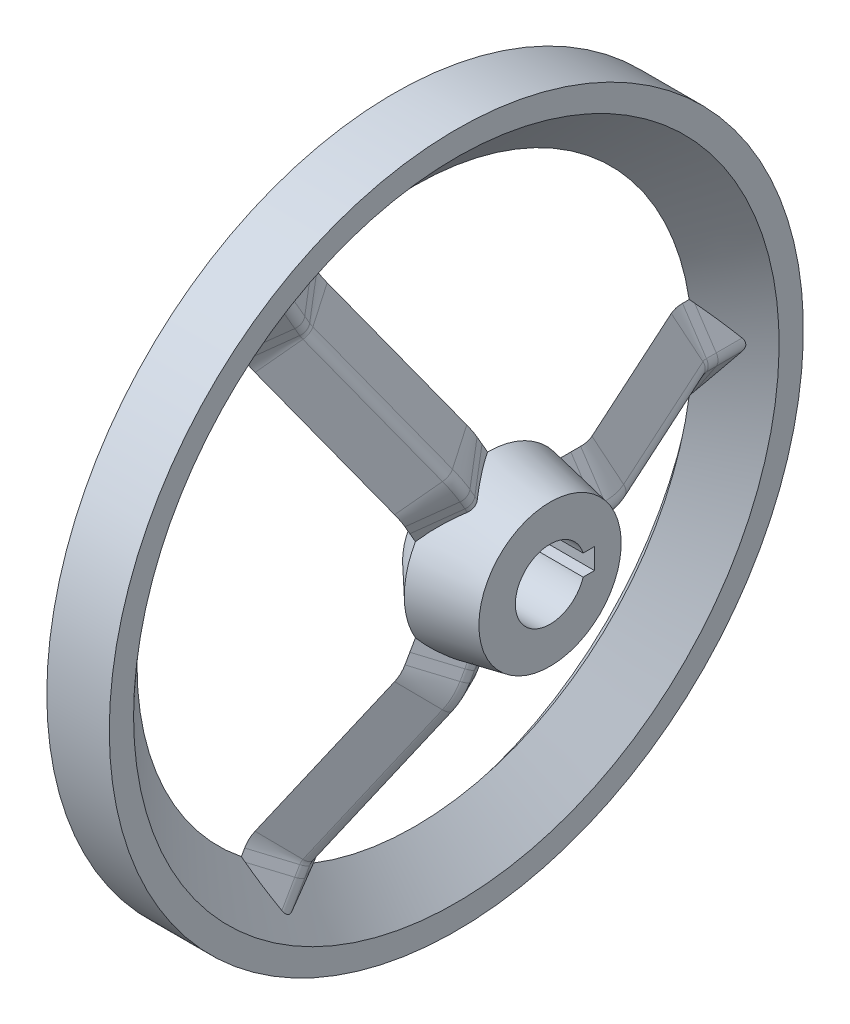
SolidWorks part; units mm, degrees
ref_plane "前视基准面" through (0, 0, 0) normal (0, 0, 1) x (1, 0, 0)
ref_plane "上视基准面" through (0, 0, 0) normal (0, 1, 0) x (1, 0, 0)
ref_plane "右视基准面" through (0, 0, 0) normal (1, 0, 0) x (0, 0, -1)
other "Configuration Table"
sketch "草图1" plane through (0, 0, 0) normal (0, 0, 1) x (1, 0, 0)
  line L0 (0, 0) -> (121.4845, 0) construction
  line L1 (0, 100) -> (0, 87.5)
  line L2 (0, 87.5) -> (6, 80)
  line L3 (6, 80) -> (18, 93)
  line L4 (18, 93) -> (18, 100)
  line L5 (18, 100) -> (0, 100)
  line L7 (27, 24) -> (45, 20.5)
  line L8 (45, 20.5) -> (45, 10)
  line L9 (45, 10) -> (18, 10)
  line L10 (18, 10) -> (18, 15.5)
  line L11 (18, 15.5) -> (27, 24)
  point P10 (18, 96.5)
  dimension "D1" = 12.5
  dimension "D2" = 18
  dimension "D3" = 6
  dimension "D4" = 7
  dimension "D5" = 200
  dimension "D6" = 27
  dimension "D7" = 48
  dimension "D8" = 160
  dimension "D9" = 20
  dimension "D10" = 10.5
  dimension "D11" = 9
  dimension "D12" = 5.5
  dimension "D13" = 45
revolve "旋转1" add sketch "草图1" angle 360 about L0
ref_plane "基准面1" through (0, 0, -14) normal (0, 0, 1) x (1, 0, 0)
sketch "草图2" plane through (0, 0, -14) normal (0, 0, 1) x (1, 0, 0)
  line L0 (0, 0) -> (44.3337, 0) construction
  line L6 (27, 12) -> (22.4808, 1.1538)
  line L7 (22.4808, -1.1538) -> (27, -12)
  line L8 (27, -24) -> (27, 24) construction
  line L9 (27, -12) -> (33.8906, -1.6641)
  line L10 (33.8906, 1.6641) -> (27, 12)
  arc A0 (33.8906, -1.6641) -> (33.8906, 1.6641) centre (31.3944, 0) ccw
  arc A1 (22.4808, 1.1538) -> (22.4808, -1.1538) centre (25.25, 0) ccw
  point P17 (35, 0)
  point P20 (22, 0)
  dimension "D1" = 13
  dimension "D2" = 24
  dimension "D5" = 3
  dimension "D3" = 5
  dimension "D4" = 12
sketch "草图3" plane through (0, 0, 0) normal (0, 1, 0) x (1, 0, 0)
  line L0 (26.0969, 30.9783) -> (6.9031, 73.0217)
  line L1 (6, 77.1747) -> (6, 80)
  line L2 (27, -24) -> (27, 24) construction
  line L3 (6, -100) -> (6, 100) construction
  line L4 (0, -100) -> (18, -100) construction
  line L5 (18, 100) -> (0, 100) construction
  line L6 (27, 24) -> (27, 14)
  line L7 (27, 26.8253) -> (27, 24)
  line L8 (6, 80) -> (6, 90)
  line L9 (45, -20.5) -> (45, 20.5) construction
  line L11 (0, 100) -> (0, -100) construction
  arc A0 (26.0969, 30.9783) -> (27, 26.8253) centre (17, 26.8253) cw
  arc A1 (6, 77.1747) -> (6.9031, 73.0217) centre (16, 77.1747) ccw
  point P22 (27, 29)
  point P25 (6, 75)
  dimension "D8" = 10
  dimension "D1" = 10
  dimension "D2" = 15
  dimension "D3" = 5
  dimension "D4" = 15
  dimension "D5" = 6
  dimension "D6" = 10
  dimension "D7" = 14
  dimension "D9" = 18
sweep "扫描4" add profiles "草图2" path "草图3"
pattern_circular "阵列(圆周)1" count 3 over 360 about axis through (0, 0, 0) along (1, 0, 0) of "扫描4"
ref_plane "基准面2" through (6, 0, 0) normal (-1, 0, 0) x (0, 0, 1)
sketch "草图4" plane through (6, 0, 0) normal (-1, 0, 0) x (0, 0, 1)
  line L1 (0, 0) -> (42.0474, 72.8283) construction
  line L2 (0, 0) -> (0, 48.3174) construction
  circle A0 centre (42.0474, 72.8283) radius 13
  dimension "D1" = 26
  dimension "D3" = 30
  dimension "D2" = 84.0949
extrude "凸台-拉伸1" add sketch "草图4" along normal up to surface (6 mm away) up to face at (0, 0, 87.5)
sketch "草图5" plane through (6, 0, 0) normal (-1, 0, 0) x (0, 0, 1)
  line L1 (-12.8, -3) -> (-7.8, -3)
  line L2 (-12.8, -3) -> (-12.8, 3)
  line L3 (-12.8, 3) -> (-7.8, 3)
  line L4 (-7.8, -3) -> (-7.8, 3)
  line L5 (-10.3, 3) -> (-10.3, -3) construction
  line L6 (-12.8, 0) -> (-7.8, 0) construction
  point P0 (-10.3, 0)
  dimension "D1" = 5
  dimension "D2" = 6
  dimension "D3" = 12.8
  dimension "D4" = 3
extrude "切除-拉伸1" cut sketch "草图5" against normal through all
